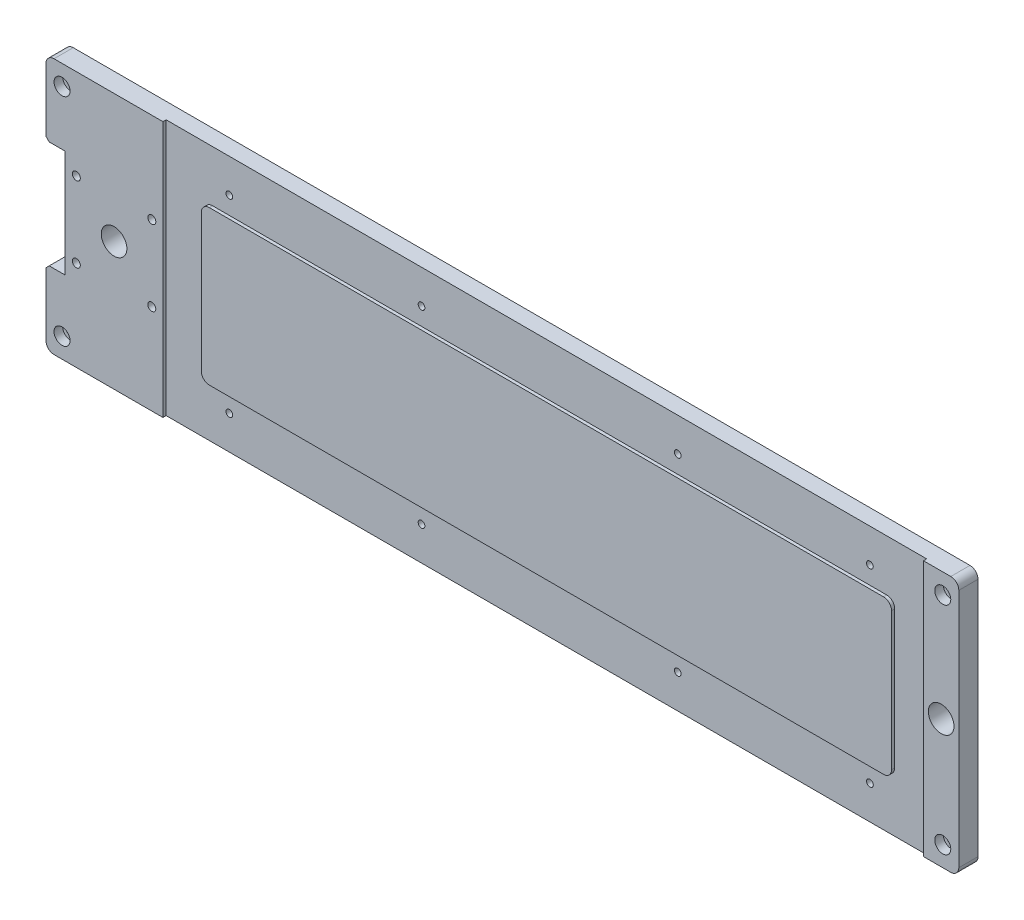
SolidWorks part; units mm, degrees
ref_plane "Front Plane" through (0, 0, 0) normal (0, 0, 1) x (1, 0, 0)
ref_plane "Top Plane" through (0, 0, 0) normal (0, 1, 0) x (1, 0, 0)
ref_plane "Right Plane" through (0, 0, 0) normal (1, 0, 0) x (0, 0, -1)
sketch "Sketch1" plane through (0, 0, 0) normal (0, 0, 1) x (1, 0, 0)
  line L1 (-285, -80) -> (285, -80)
  line L2 (-285, -80) -> (-285, 80)
  line L3 (-285, 80) -> (285, 80)
  line L4 (285, -80) -> (285, 80)
  line L5 (-285, -80) -> (285, 80) construction
  line L6 (-285, 80) -> (285, -80) construction
  point P0 (0, 0)
  dimension "D1" = 570
  dimension "D2" = 160
extrude "Boss-Extrude1" add sketch "Sketch1" along normal blind 12
sketch "Sketch2" plane through (0, 0, 12) normal (0, 0, 1) x (1, 0, 0)
  line L0 (-285, 80) -> (-285, -80) construction
  line L1 (-212, 112.7786) -> (-188, 112.7786)
  line L2 (-212, 112.7786) -> (-212, -133.7282)
  line L3 (-212, -133.7282) -> (-188, -133.7282)
  line L4 (-188, 112.7786) -> (-188, -133.7282)
  line L5 (243, 121.1584) -> (263, 121.1584)
  line L6 (243, 121.1584) -> (243, -139.3148)
  line L7 (243, -139.3148) -> (263, -139.3148)
  line L8 (263, 121.1584) -> (263, -139.3148)
  dimension "D1" = 24
  dimension "D2" = 97
  dimension "D3" = 431
  dimension "D4" = 20
extrude "Cut-Extrude1" cut sketch "Sketch2" against normal blind 2
sketch "Sketch3" plane through (0, 0, 12) normal (0, 0, 1) x (1, 0, 0)
  line L0 (243, 80) -> (243, -80) construction
  line L1 (-188, 80) -> (243, 80)
  line L2 (-188, 80) -> (-188, 48)
  line L3 (-188, 48) -> (243, 48)
  line L4 (243, 80) -> (243, 48)
  line L5 (0, 0) -> (91.3788, 0) construction
  line L6 (243, -80) -> (243, -48)
  line L7 (-188, -48) -> (243, -48)
  line L8 (-188, -80) -> (-188, -48)
  line L9 (-188, -80) -> (243, -80)
  dimension "D1" = 32
extrude "Cut-Extrude2" cut sketch "Sketch3" against normal blind 2
sketch "Sketch4" plane through (0, 0, 12) normal (0, 0, 1) x (1, 0, 0)
  line L0 (-285, 80) -> (-285, -80) construction
  line L1 (-285, 33.5) -> (-273, 33.5)
  line L2 (-285, 33.5) -> (-285, -33.5)
  line L3 (-285, -33.5) -> (-273, -33.5)
  line L4 (-273, 33.5) -> (-273, -33.5)
  line L5 (0, 0) -> (-273, 0) construction
  dimension "D1" = 12
  dimension "D2" = 67
extrude "Cut-Extrude3" cut sketch "Sketch4" against normal through all
hole_wizard "M5 Tapped Hole1" positions "Sketch9" profile "Sketch10" tap size "M5" standard "ISO" end condition through all
sketch "Sketch9" plane through (0, 0, 10) normal (0, 0, 1) x (1, 0, 0)
  point P0 (227.5, -59)
  point P3 (107.5, -59)
  point P6 (-172.5, -59)
  point P9 (-52.5, -59)
  point P12 (-172.5, 59)
  point P15 (-52.5, 59)
  point P18 (107.5, 59)
  point P21 (227.5, 59)
sketch "Sketch10" plane through (227.5, -59, 10) normal (1, 0, 0) x (0, -1, 0)
  line L0 (0, 0) -> (0, 10)
  line L1 (0, 10) -> (2.1, 10)
  line L2 (2.1, 10) -> (2.1, 0)
  line L5 (2.1, 0) -> (0, 0)
  line L11 (0, -6.35) -> (0, 107.95) construction
  dimension "通孔螺纹孔钻头直径" = 4.2
  dimension "通孔螺纹孔钻头深度" = 10
cosmetic thread "Cosmetic Thread7" parameters "D2"=5
cosmetic thread "Cosmetic Thread8" parameters "D2"=5
cosmetic thread "Cosmetic Thread9" parameters "D2"=5
cosmetic thread "Cosmetic Thread10" parameters "D2"=5
cosmetic thread "Cosmetic Thread11" parameters "D2"=5
cosmetic thread "Cosmetic Thread12" parameters "D2"=5
cosmetic thread "Cosmetic Thread13" parameters "D2"=5
cosmetic thread "Cosmetic Thread14" parameters "D2"=5
fillet "Fillet1" radius 5 4 edges at (-188, -48, 11) (-188, 48, 11) (243, -48, 11) (243, 48, 11)
fillet "Fillet2" radius 5 4 edges at (-285, 80, 6) (-285, -80, 6) (285, -80, 6) (285, 80, 6)
chamfer "Chamfer1" distance 2 angle 45 2 edges at (-285, 33.5, 6) (-285, -33.5, 6)
hole_wizard "CBORE for M5 Hex Socket Head Cap Screw1" positions "Sketch11" profile "Sketch12" counterbore size "M5" standard "ISO" end condition through all
sketch "Sketch11" plane through (0, 0, 12) normal (0, 0, 1) x (1, 0, 0)
  line L1 (-275, -67.5) -> (275, -67.5) construction
  line L2 (-275, -67.5) -> (-275, 67.5) construction
  line L3 (-275, 67.5) -> (275, 67.5) construction
  line L4 (275, -67.5) -> (275, 67.5) construction
  line L5 (-275, -67.5) -> (275, 67.5) construction
  line L6 (-275, 67.5) -> (275, -67.5) construction
  line L7 (285, -75) -> (285, 75) construction
  point P2 (275, 67.5)
  point P5 (-275, -67.5)
  point P6 (-275, 67.5)
  point P7 (275, -67.5)
  dimension "D1" = 10
  dimension "D2" = 135
sketch "Sketch12" plane through (275, 67.5, 12) normal (1, 0, 0) x (0, -1, 0)
  line L0 (0, 0) -> (0, 12)
  line L1 (0, 12) -> (2.75, 12)
  line L3 (2.75, 12) -> (2.75, 5.4)
  line L4 (2.75, 5.4) -> (5, 5.4)
  line L5 (5, 5.4) -> (5, 0)
  line L7 (5, 0) -> (0, 0)
  line L11 (0, -6.35) -> (0, 107.95) construction
  dimension "通孔孔直径" = 5.5
  dimension "通孔孔深度" = 12
  dimension "柱形沉头孔直径" = 10
  dimension "柱形沉头孔深度" = 5.4
sketch "Sketch13" plane through (0, 0, 12) normal (0, 0, 1) x (1, 0, 0)
  line L0 (-273, 0) -> (-212, 0) construction
  line L2 (-273, -33.5) -> (-273, 33.5) construction
  line L3 (-212, 80) -> (-212, -80) construction
  circle A0 centre (-242.5, 0) radius 8
extrude "Cut-Extrude4" cut sketch "Sketch13" against normal blind 18
sketch "Sketch14" plane through (0, 0, 0) normal (0, 0, -1) x (-1, 0, 0)
  circle A0 centre (218.93, -23.57) radius 2.5 construction
  circle A1 centre (266.07, -23.57) radius 2.5 construction
  circle A2 centre (266.07, 23.57) radius 2.5 construction
  circle A3 centre (218.93, 23.57) radius 2.5 construction
  circle A4 centre (218.93, -23.57) radius 2.5
  circle A5 centre (266.07, -23.57) radius 2.5
  circle A6 centre (266.07, 23.57) radius 2.5
  circle A7 centre (218.93, 23.57) radius 2.5
extrude "Cut-Extrude5" cut sketch "Sketch14" against normal up to surface (12 mm away) up to face at (-234.5, 0, 12)
sketch "Sketch15" plane through (0, 0, 12) normal (0, 0, 1) x (1, 0, 0)
  line L0 (263, 0) -> (285, 0) construction
  line L1 (263, 80) -> (263, -80) construction
  line L2 (285, -75) -> (285, 75) construction
  circle A0 centre (274, 0) radius 8
extrude "Cut-Extrude6" cut sketch "Sketch15" against normal up to surface (12 mm away) up to face at (-221.43, 23.57, 0)
